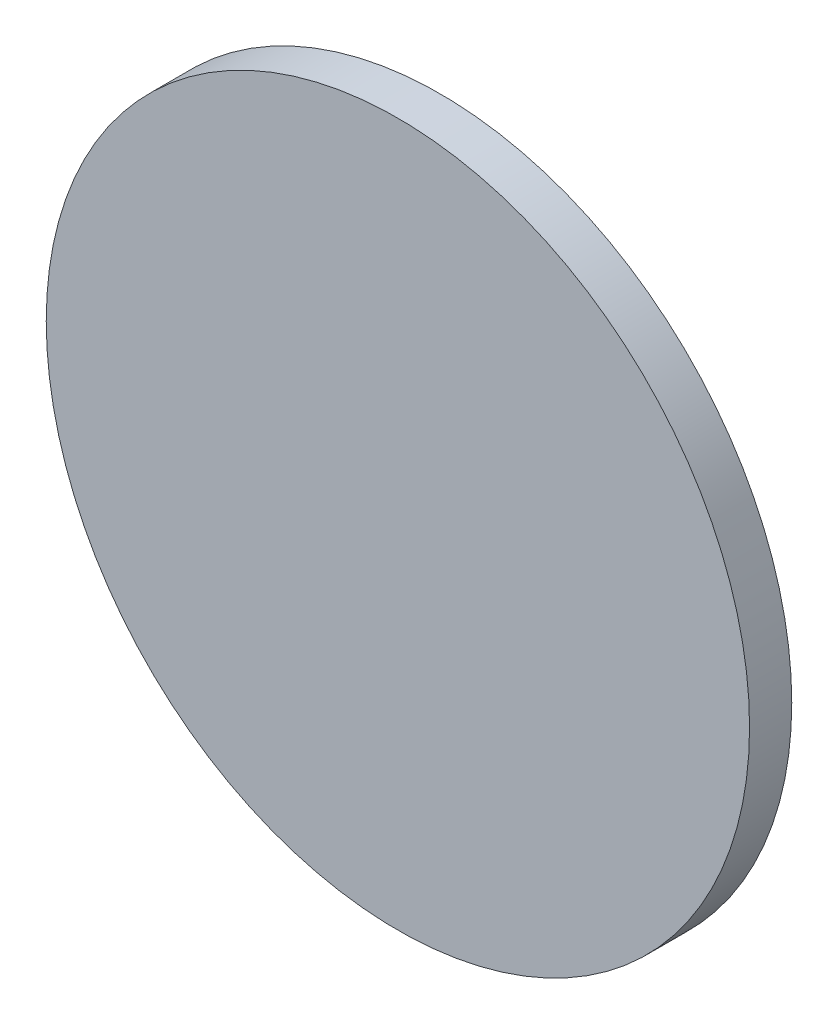
SolidWorks part; units mm, degrees
ref_plane "Front Plane" through (0, 0, 0) normal (0, 0, 1) x (1, 0, 0)
ref_plane "Top Plane" through (0, 0, 0) normal (0, 1, 0) x (1, 0, 0)
ref_plane "Right Plane" through (0, 0, 0) normal (1, 0, 0) x (0, 0, -1)
sketch "Sketch1" plane through (0, 0, 0) normal (0, 0, 1) x (1, 0, 0)
  circle A0 centre (0, 0) radius 25
  dimension "D1" = 50
extrude "Boss-Extrude1" add sketch "Sketch1" along normal blind 3
